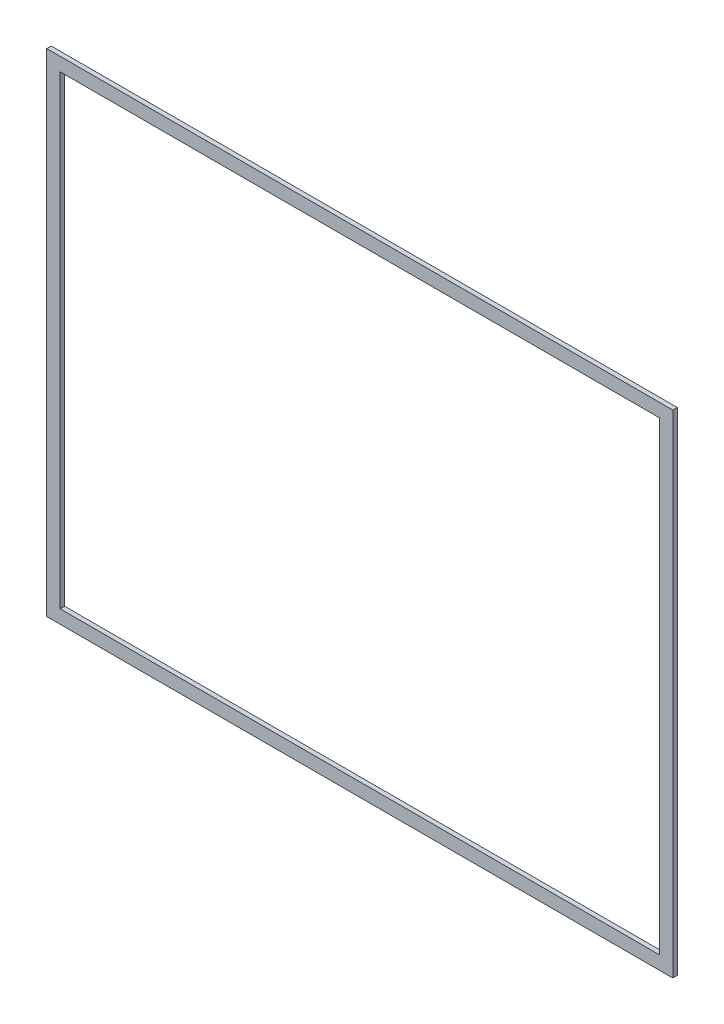
SolidWorks part; units mm, degrees
ref_plane "前视基准面" through (0, 0, 0) normal (0, 0, 1) x (1, 0, 0)
ref_plane "上视基准面" through (0, 0, 0) normal (0, 1, 0) x (1, 0, 0)
ref_plane "右视基准面" through (0, 0, 0) normal (1, 0, 0) x (0, 0, -1)
other "Configuration Table"
sketch "草图1" plane through (0, 0, 0) normal (0, 0, 1) x (1, 0, 0)
  line L0 (-70, -55) -> (70, -55)
  line L1 (70, -55) -> (70, 55)
  line L2 (70, 55) -> (-70, 55)
  line L3 (-70, 55) -> (-70, -55)
  line L4 (-67, -52) -> (67, -52)
  line L5 (67, -52) -> (67, 52)
  line L6 (67, 52) -> (-67, 52)
  line L7 (-67, 52) -> (-67, -52)
  point P0 (0, 0)
  dimension "D1" = 3
  dimension "D2" = 70
  dimension "D3" = 137
  dimension "D4" = 140
  dimension "D5" = 3
  dimension "D6" = 55
  dimension "D7" = 107
  dimension "D8" = 110
extrude "凸台-拉伸1" add sketch "草图1" against normal mid plane 1
